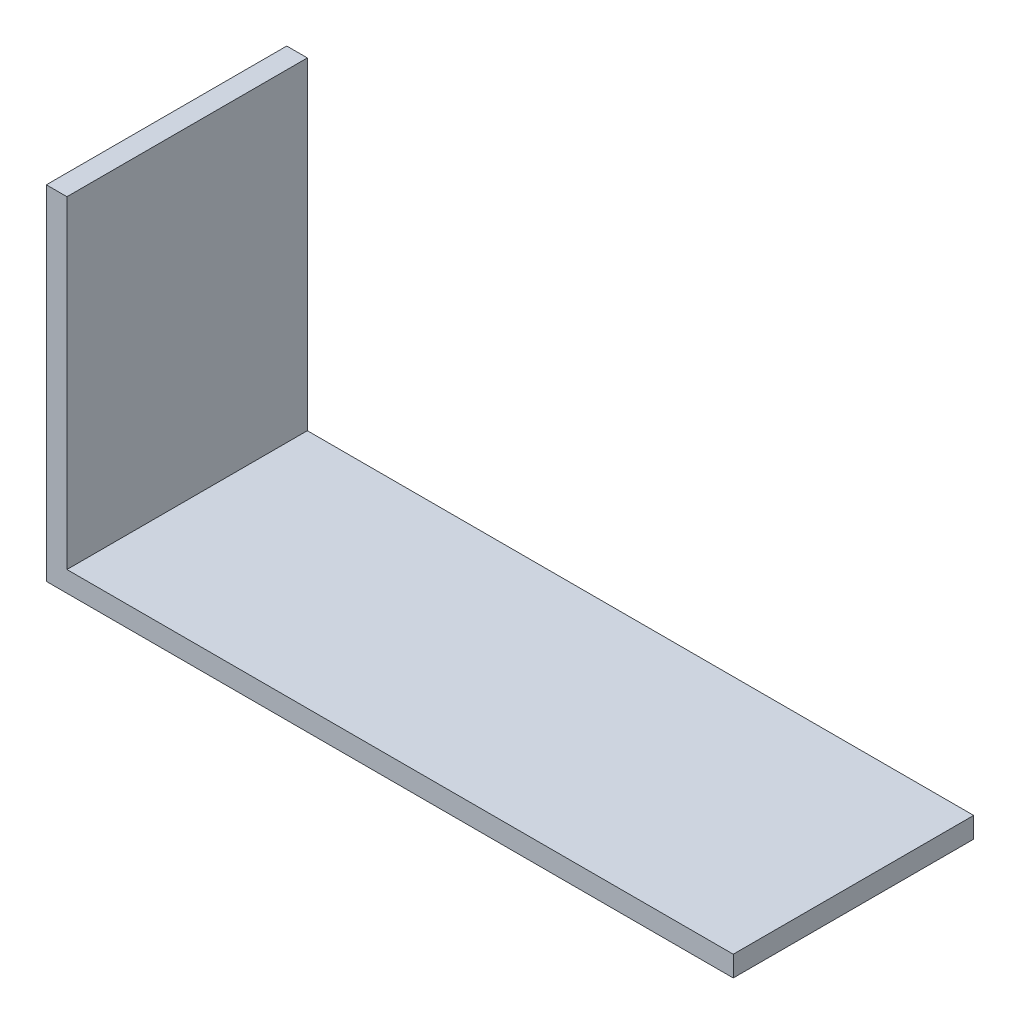
SolidWorks part; units mm, degrees
ref_plane "前视基准面" through (0, 0, 0) normal (0, 0, 1) x (1, 0, 0)
ref_plane "上视基准面" through (0, 0, 0) normal (0, 1, 0) x (1, 0, 0)
ref_plane "右视基准面" through (0, 0, 0) normal (1, 0, 0) x (0, 0, -1)
sketch "草图1" plane through (0, 0, 0) normal (0, 0, 1) x (1, 0, 0)
  line L0 (0, 0) -> (0, -100)
  line L1 (0, -100) -> (200, -100)
  line L2 (6, 0) -> (6, -94)
  line L3 (6, -94) -> (200, -94)
  line L4 (0, 0) -> (6, 0)
  line L5 (200, -100) -> (200, -94)
  dimension "D1" = 6
extrude "凸台-拉伸1" add sketch "草图1" along normal blind 70
